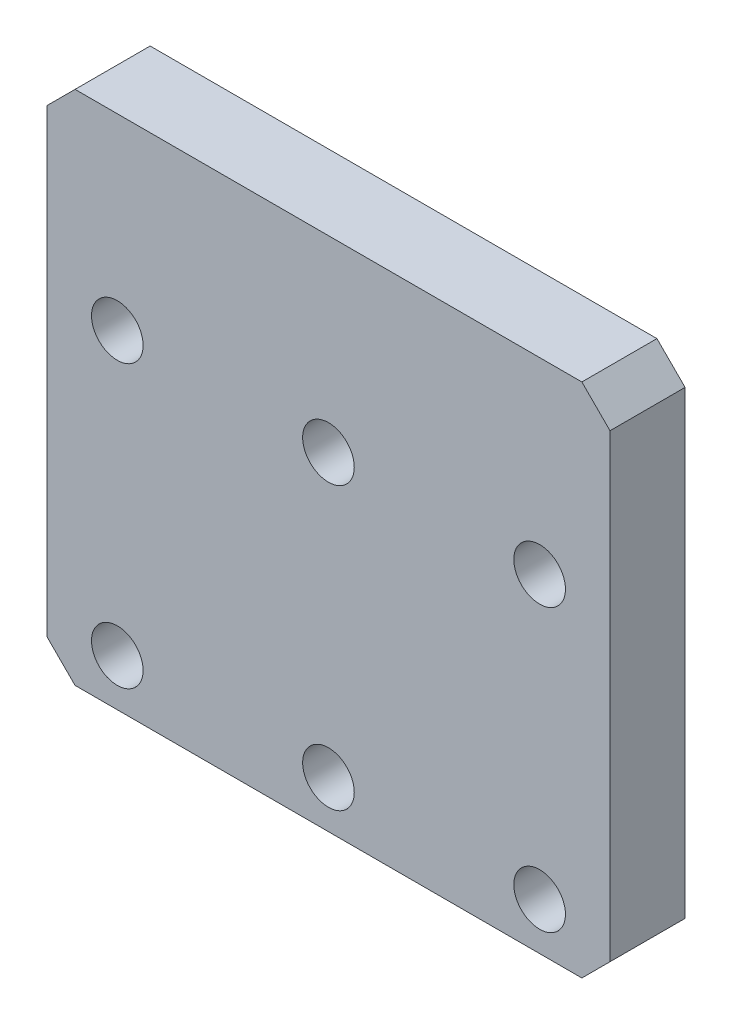
from build123d import *

# Parameters (mm, degrees)
SKETCH1_W                  = 60
SKETCH1_H                  = 55
BOSS_EXTRUDE1_DEPTH        = 8
F_5_5_5_5_DIAMETER_HOLE1_D = 5.5
CHAMFER1_SIZE              = 3


with BuildPart() as part:
    # Sketch1 → Boss-Extrude1 (new body)
    with BuildSketch(Plane.XY):
        Rectangle(SKETCH1_W, SKETCH1_H)
    extrude(amount=BOSS_EXTRUDE1_DEPTH)

    # Ø5.5 (5.5) Diameter Hole1 (through all)
    with Locations(Plane.XY.offset(8)):
        with Locations((-22.5, -22.5), (-22.5, 7.5), (0, 7.5), (0, -22.5), (22.5, -22.5), (22.5, 7.5)):
            Hole(F_5_5_5_5_DIAMETER_HOLE1_D / 2)

    # Chamfer1
    chamfer1_edges = [part.edges().sort_by_distance(p)[0] for p in [
        (30, -27.5, 4),
        (-30, -27.5, 4),
        (-30, 27.5, 4),
        (30, 27.5, 4),
    ]]
    chamfer(chamfer1_edges, length=CHAMFER1_SIZE)


solid = part.part
